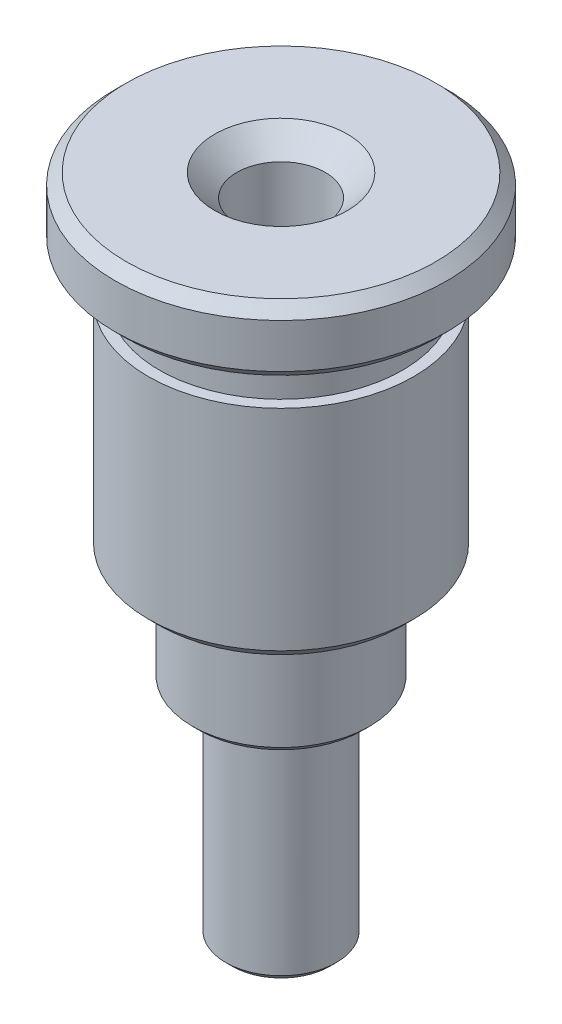
from build123d import *

# Parameters (mm, degrees)
SKETCH_1_R          = 6
EXTRUDE_1_DEPTH     = 15
SKETCH_2_R          = 2.5
EXTRUDE_2_DEPTH     = 15
SKETCH_3_R          = 2
CUT_EXTRUDE_1_DEPTH = 32.176914536
CHAMFER_2_SIZE      = 0.5
SKETCH_6_R          = 7.5
SKETCH_6_R_2        = 6
EXTRUDE_3_DEPTH     = 3
CHAMFER_3_SIZE      = 1
CHAMFER_4_SIZE      = 0.5
SKETCH_7_R          = 4
SKETCH_7_R_2        = 2.5
EXTRUDE_4_DEPTH     = 5
CHAMFER_5_SIZE      = 0.3
CHAMFER_6_SIZE      = 0.3
SKETCH_8_W          = 3.367745964
SKETCH_8_H          = 2


with BuildPart() as part:
    # 草图1 → 凸台-拉伸1 (new body)
    with BuildSketch(Plane(origin=(0, 0, 0), x_dir=(1, 0, 0), z_dir=(0, 1, 0))):
        with Locations(Location((0, 0, 0), (0, 0, 270))):
            Circle(SKETCH_1_R)
    extrude(amount=-EXTRUDE_1_DEPTH)

    # 草图2 → 凸台-拉伸2 (add)
    with BuildSketch(Plane.XZ.offset(15)):
        with Locations(Location((0, 0, 0), (0, 0, 90))):
            Circle(SKETCH_2_R)
    extrude(amount=EXTRUDE_2_DEPTH)

    # 草图3 → 切除-拉伸1 (cut, through all)
    with BuildSketch(Plane(origin=(0, 0, 0), x_dir=(1, 0, 0), z_dir=(0, 1, 0))):
        with Locations(Location((0, 0, 0), (0, 0, 270))):
            Circle(SKETCH_3_R)
    extrude(amount=-CUT_EXTRUDE_1_DEPTH, mode=Mode.SUBTRACT)

    # 倒角2
    chamfer_2_edges = [part.edges().sort_by_distance(p)[0] for p in [
        (0, -15, -6),
    ]]
    chamfer(chamfer_2_edges, length=CHAMFER_2_SIZE)

    # 草图6 → 凸台-拉伸3 (add)
    with BuildSketch(Plane(origin=(0, 0, 0), x_dir=(1, 0, 0), z_dir=(0, 1, 0))):
        with Locations(Location((0, 0, 0), (0, 0, 270))):
            Circle(SKETCH_6_R)
        with Locations(Location((0, 0, 0), (0, 0, 270))):
            Circle(SKETCH_6_R_2, mode=Mode.SUBTRACT)
    extrude(amount=-EXTRUDE_3_DEPTH)

    # 倒角3
    chamfer_3_edges = [part.edges().sort_by_distance(p)[0] for p in [
        (0, 0, -2),
    ]]
    chamfer(chamfer_3_edges, length=CHAMFER_3_SIZE)

    # 倒角4
    chamfer_4_edges = [part.edges().sort_by_distance(p)[0] for p in [
        (0, -3, -7.5),
        (0, 0, -7.5),
    ]]
    chamfer(chamfer_4_edges, length=CHAMFER_4_SIZE)

    # 草图7 → 凸台-拉伸4 (add)
    with BuildSketch(Plane.XZ.offset(15)):
        with Locations(Location((0, 0, 0), (0, 0, 90))):
            Circle(SKETCH_7_R)
        with Locations(Location((0, 0, 0), (0, 0, 270))):
            Circle(SKETCH_7_R_2, mode=Mode.SUBTRACT)
    extrude(amount=EXTRUDE_4_DEPTH)

    # 倒角5
    chamfer_5_edges = [part.edges().sort_by_distance(p)[0] for p in [
        (0, -20, -4),
    ]]
    chamfer(chamfer_5_edges, length=CHAMFER_5_SIZE)

    # 倒角6
    chamfer_6_edges = [part.edges().sort_by_distance(p)[0] for p in [
        (0, -30, -2.5),
    ]]
    chamfer(chamfer_6_edges, length=CHAMFER_6_SIZE)

    # 草图8 → 切除-旋转1 (revolve, cut)
    with BuildSketch(Plane.XY, mode=Mode.PRIVATE) as cut_revolve_1_sk:
        with Locations((-7.183872982, -4)):
            Rectangle(SKETCH_8_W, SKETCH_8_H)
    revolve(cut_revolve_1_sk.sketch.rotate(Axis((0, -15, 0), (0, 1, 0)), 90), axis=Axis((0, -15, 0), (0, 1, 0)), mode=Mode.SUBTRACT)


solid = part.part
